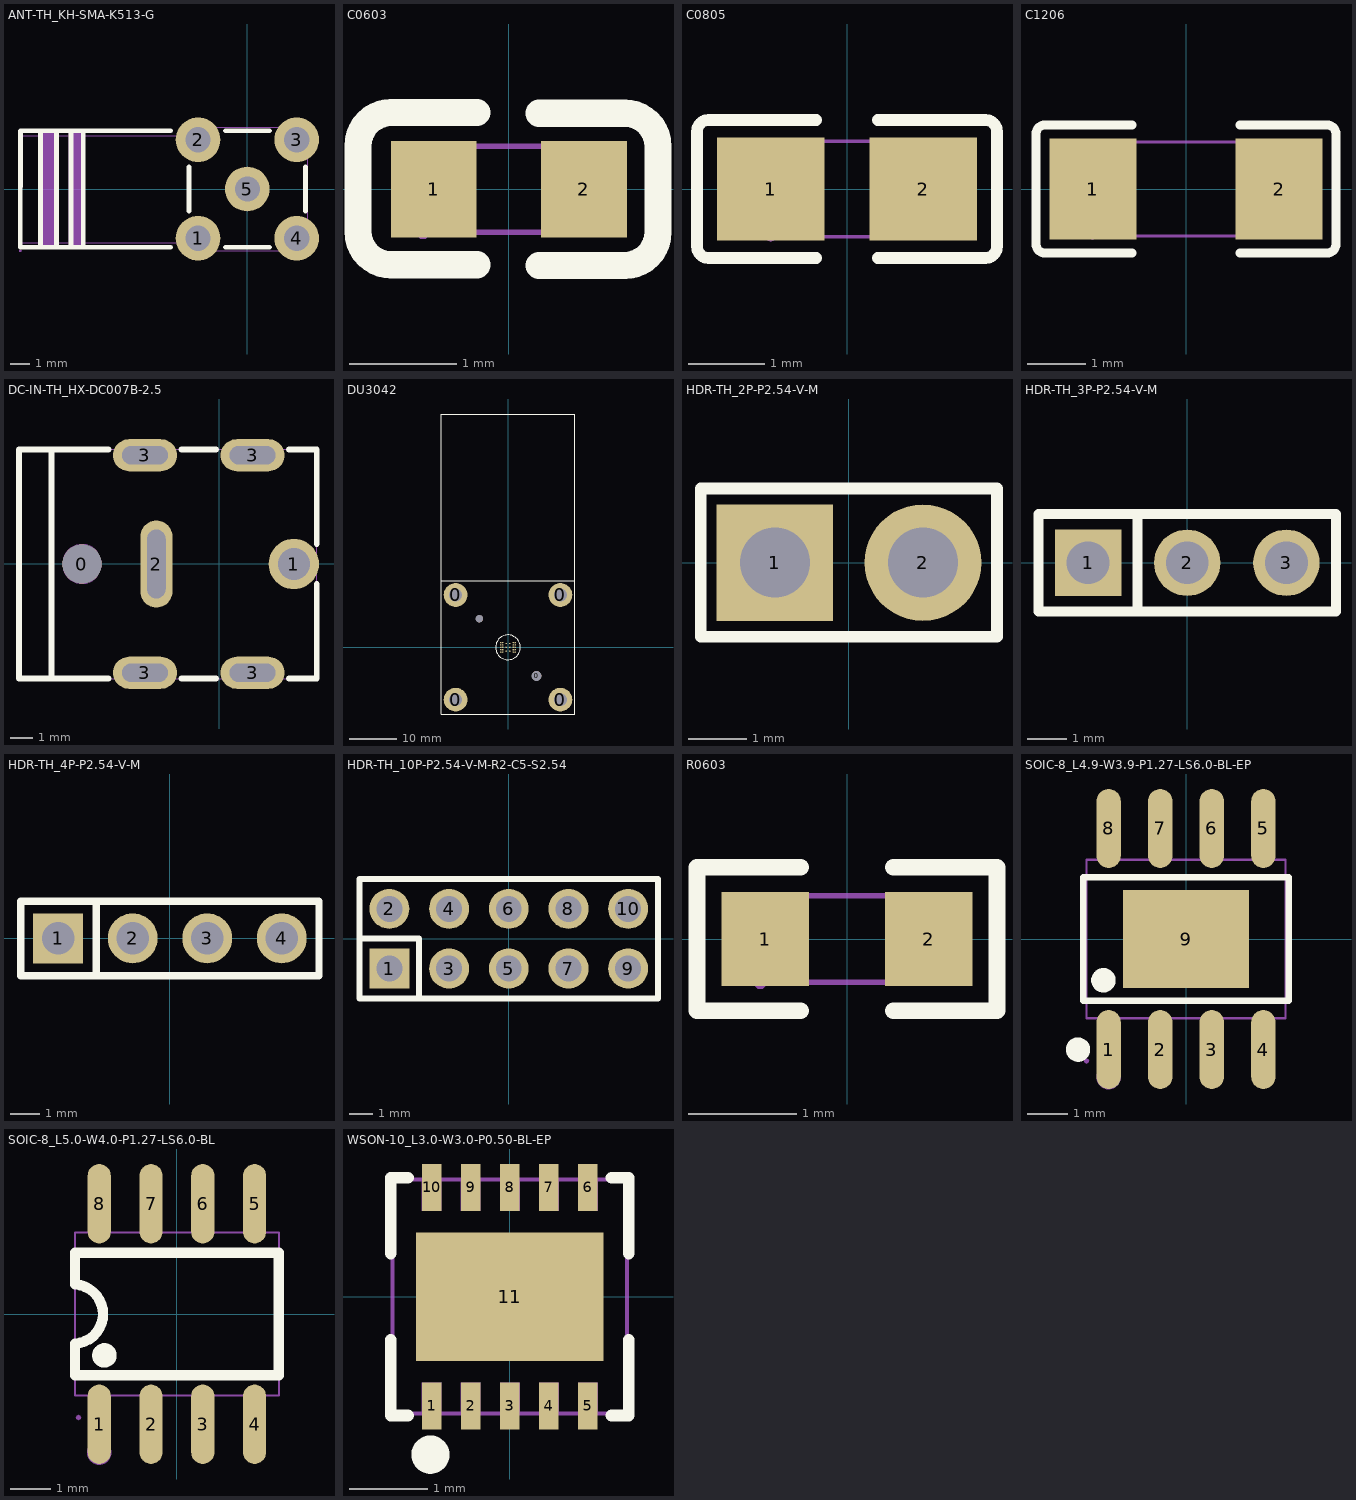
[diagram p0: the footprints below, top view; thin cyan lines are the x and y axes]
# Altium footprint library MISC75514.PcbLib: 14 footprints
Each footprint in its own frame and in the unit in brackets; x right, y up, seen from the top. Pads: shape width x height; smd on the part's side, far side on the other; paste and mask are expansions set on the pad; w line width, h text height; cw(c..) or ccw(c..) is an arc to the next point about the centre after c.

## ANT-TH_KH-SMA-K513-G [mm]
height 1.4
pads (5):
  round 2.3 hole 1.3 paste+0.051: 1(-2.54,-2.54) 2(-2.54,2.54) 3(2.54,2.54) 4(2.54,-2.54) 5(0,0)
Top Overlay:
  lines w0.254: -11.69,2.98 -11.7,-2.83 -11.7,-3 -11.5,-3 -3.948,-3 ; -11.69,3 -11.361,3 ; -11.5,3 -3.948,3 ; -10.668,-3 -10.668,3 ; -9.966,3 -9.573,3 ; -9.827,-3 -9.827,3 ; -9.09,-3 -9.09,3 ; -8.595,3 -8.176,3 ; -8.455,-3 -8.455,3 ; -3,-1.132 -3,1.132 ; -1.132,-3 1.132,-3 ; -1.132,3 1.132,3 ; 3,-1.132 3,1.132
Mechanical 2:
  region: -9.194,2.972 -8.394,2.972 -8.394,-3.018 -8.404,-3.028 -9.204,-3.028
  region: -10.64,3 -9.84,3 -9.84,-2.99 -9.85,-3 -10.65,-3
Mechanical 6:
  lines w0.051: -11.7,-2.76 -3.25,-2.76 -3.25,-3.17 3.1,-3.18 3.1,3.17 -3.25,3.17 -3.25,2.75 -11.7,2.75 -11.7,-2.76
Mechanical 8:
  region: -11.635,-3.18 -11.654,-3.226 -11.7,-3.245 -11.746,-3.226 -11.765,-3.18 -11.746,-3.134 -11.7,-3.115 -11.654,-3.134
Mechanical 9:
  region: -2.99,-2.09 -2.09,-2.09 -2.09,-2.99 -2.99,-2.99
  region: 2.09,2.99 2.99,2.99 2.99,2.09 2.09,2.09
  region: -2.99,2.99 -2.09,2.99 -2.09,2.09 -2.99,2.09
  region: 2.09,-2.09 2.99,-2.09 2.99,-2.99 2.09,-2.99
  region: 0.408,0 0.377,-0.156 0.288,-0.288 0.156,-0.377 0,-0.408 -0.156,-0.377 -0.288,-0.288 -0.377,-0.156 -0.408,0 -0.377,0.156 -0.288,0.288 -0.156,0.377 0,0.408 0.156,0.377 0.288,0.288 0.377,0.156

## C0603 [mm]
height 1.4
pads (2):
  rect 0.8x0.9 smd: 1(-0.7,0) 2(0.7,0)
Top Overlay:
  lines w0.254: -0.296,-0.704 -1.096,-0.704 cw(c-1.096,-0.394) -1.406,-0.394 -1.405,0.406 cw(c-1.096,0.406) -1.096,0.715 -0.296,0.715 ; 0.28,-0.71 1.08,-0.71 ccw(c1.08,-0.4) 1.39,-0.4 1.39,0.4 ccw(c1.08,0.4) 1.08,0.71 0.28,0.71
Mechanical 15:
  region: -0.8,-0.4 -0.8,0.4 -0.5,0.4 -0.5,-0.4
  region: 0.8,-0.4 0.8,0.4 0.5,0.4 0.5,-0.4
  region: -0.74,-0.4 -0.74,-0.375 -0.775,-0.341 -0.825,-0.341 -0.86,-0.375 -0.86,-0.4 -0.86,-0.425 -0.825,-0.459 -0.776,-0.459 -0.741,-0.425 -0.74,-0.4
  lines w0.051: -0.8,-0.4 -0.8,0.4 0.8,0.4 0.8,-0.4 -0.8,-0.4

## C0805 [mm]
height 1.4
pads (2):
  rect 1.41x1.35 smd paste-100 mask+0.051: 1(-1,0) 2(1,0)
Top Overlay:
  lines w0.152: -0.401,-0.904 -1.811,-0.904 cw(c-1.811,-0.751) -1.964,-0.751 -1.964,0.751 cw(c-1.811,0.751) -1.811,0.904 -0.401,0.904 ; 0.401,-0.904 1.811,-0.904 ccw(c1.811,-0.751) 1.964,-0.751 1.964,0.751 ccw(c1.811,0.751) 1.811,0.904 0.401,0.904
Top Paste:
  region: -1.705,-0.64 -1.705,0.64 -1.655,0.69 -0.505,0.69 -0.455,0.64 -0.45,0.23 -0.9,0.23 -0.9,-0.22 -0.46,-0.22 -0.455,-0.64 -0.505,-0.69 -1.655,-0.69
  region: 1.705,0.64 1.705,-0.64 1.655,-0.69 0.505,-0.69 0.455,-0.64 0.45,-0.23 0.9,-0.23 0.9,0.22 0.46,0.22 0.455,0.64 0.505,0.69 1.655,0.69
Mechanical 6:
  lines w0.051: -1,-0.625 -1,0.625 1,0.625 1,-0.625 -1,-0.625
Mechanical 8:
  region: -0.935,-0.625 -0.954,-0.671 -1,-0.69 -1.046,-0.671 -1.065,-0.625 -1.046,-0.579 -1,-0.56 -0.954,-0.579
Mechanical 9:
  region: -1,-0.625 -1,0.625 -0.5,0.625 -0.5,-0.625
  region: 1,0.625 1,-0.625 0.5,-0.625 0.5,0.625

## C1206 [mm]
height 1.4
pads (2):
  rect 1.485x1.728 smd paste-100 mask+0.051: 1(-1.593,0) 2(1.593,0)
Top Overlay:
  lines w0.152: -0.926,-1.093 -2.411,-1.093 cw(c-2.411,-0.94) -2.564,-0.94 -2.564,0.94 cw(c-2.411,0.94) -2.411,1.093 -0.926,1.093 ; 0.926,-1.093 2.411,-1.093 ccw(c2.411,-0.94) 2.564,-0.94 2.564,0.94 ccw(c2.411,0.94) 2.411,1.093 0.926,1.093
Top Paste:
  region: 0.85,-0.764 0.85,-0.394 0.95,-0.294 1.255,-0.294 1.355,-0.194 1.355,0.194 1.255,0.294 0.95,0.294 0.85,0.394 0.85,0.764 0.95,0.864 2.235,0.864 2.335,0.764 2.335,-0.764 2.235,-0.864 0.95,-0.864
  region: -0.85,-0.764 -0.85,-0.394 -0.95,-0.294 -1.255,-0.294 -1.355,-0.194 -1.355,0.194 -1.255,0.294 -0.95,0.294 -0.85,0.394 -0.85,0.764 -0.95,0.864 -2.235,0.864 -2.335,0.764 -2.335,-0.764 -2.235,-0.864 -0.95,-0.864
Mechanical 6:
  lines w0.051: -1.6,-0.8 -1.6,0.8 1.6,0.8 1.6,-0.8 -1.6,-0.8
Mechanical 8:
  region: -1.535,-0.8 -1.554,-0.846 -1.6,-0.865 -1.646,-0.846 -1.665,-0.8 -1.646,-0.754 -1.6,-0.735 -1.554,-0.754
Mechanical 9:
  region: -1.6,-0.8 -1.6,0.8 -1.1,0.8 -1.1,-0.8
  region: 1.6,-0.8 1.6,0.8 1.1,0.8 1.1,-0.8

## DC-IN-TH_HX-DC007B-2.5 [mm]
height 1.4
pads (7):
  round 1.7 hole 1.7 unplated: 0(-6,0)
  round 2.2 hole 1.4: 1(3.25,0)
  oval 1.4x3.8 hole 0.8 slot 3 at 90 deg: 2(-2.75,0)
  oval 2.8x1.4 hole 0.8 slot 2 at 0 deg: 3(-3.25,-4.75) 3(-3.25,4.75) 3(1.45,-4.75) 3(1.45,4.75)
Top Overlay:
  lines w0.254: -7.325,-5 -7.325,5 ; -4.847,-5 -8.75,-5 -8.75,5 -4.847,5 ; -1.653,-5 -0.147,-5 ; -1.653,5 -0.147,5 ; 3.047,-5 4.25,-5 4.25,-0.877 ; 3.047,5 4.25,5 4.25,0.877
Mechanical 1:
  circle w0.005: c-6,0 r0.85
Mechanical 15:
  region: 4.31,-5 4.309,-4.976 4.274,-4.943 4.226,-4.943 4.191,-4.976 4.19,-5 4.191,-5.024 4.226,-5.058 4.274,-5.058 4.309,-5.024 4.31,-5
  region: -4.05,4.6 -4.05,4.9 -2.45,4.9 -2.45,4.6
  region: 0.65,4.6 0.65,4.9 2.25,4.9 2.25,4.6
  region: -4.05,-4.9 -4.05,-4.6 -2.45,-4.6 -2.45,-4.9
  region: 0.65,-4.9 0.65,-4.6 2.25,-4.6 2.25,-4.9
  region: -2.65,-0.8 -2.85,-0.8 -2.85,0.8 -2.65,0.8
  region: 3.85,0 3.85,0.119 3.759,0.34 3.59,0.509 3.369,0.6 3.131,0.6 2.91,0.509 2.741,0.34 2.65,0.119 2.65,0 2.65,-0.119 2.741,-0.34 2.91,-0.509 3.131,-0.6 3.369,-0.6 3.59,-0.509 3.759,-0.34 3.85,-0.119 3.85,0
  lines w0.051: -8.75,-5 4.25,-5 4.25,5 -8.75,5 -8.75,-5

## DU3042 [mm]
height 1.4
pads (32):
  round 5 hole 2.7: 0(-11,-11) 0(-11,11) 0(11,-11) 0(11,11)
  round 1.5 hole 1.6 unplated: 0(-6,6)
  round 2 hole 2.1 unplated: 0(6,-6)
  round 0.3 smd: 1(-1.5,1) 2(-1.5,0.5) 3(-1.5,0) 4(-1.5,-0.5) 5(-1.5,-1) 6(1.5,-1) 7(1.5,-0.5) 8(1.5,0) 9(1.5,0.5) 10(1.5,1) 11(-0.4,-0.8) 11(-0.4,0) 11(-0.4,0.8) 11(0.4,-0.8) 11(0.4,0) 11(0.4,0.8) NC(-1.1,-1) NC(-1.1,-0.5) NC(-1.1,0) NC(-1.1,0.5) NC(-1.1,1) NC(1.1,-1) NC(1.1,-0.5) NC(1.1,0) NC(1.1,0.5) NC(1.1,1)
Top Overlay:
  circle w0.127: c0,0 r2.6
  lines w0.127: -14,14 -14,49 14,49 14,14 ; -14,14 -14,-14 14,-14 14,14 ; -14,14 14,14

## HDR-TH_2P-P2.54-V-M [mm]
height 1.4
pads (2):
  rect 2x2 hole 1.2 paste+0.051: 1(-1.27,0)
  round 2 hole 1.2 paste+0.051: 2(1.27,0)
Top Overlay:
  lines w0.203: -2.54,-1.27 2.54,-1.27 2.54,1.27 -0.635,1.27 -2.54,1.27 -2.54,-1.27
Mechanical 6:
  lines w0.051: -2.54,-1.25 -2.54,1.25 2.54,1.25 2.54,-1.25 -2.54,-1.25
Mechanical 8:
  region: -2.475,-1.25 -2.494,-1.296 -2.54,-1.315 -2.586,-1.296 -2.605,-1.25 -2.586,-1.204 -2.54,-1.185 -2.494,-1.204
Mechanical 9:
  region: 0.95,0.32 1.59,0.32 1.59,-0.32 0.95,-0.32
  region: -1.59,0.32 -0.95,0.32 -0.95,-0.32 -1.59,-0.32

## HDR-TH_3P-P2.54-V-M [mm]
height 1.4
pads (3):
  rect 1.7x1.7 hole 1.1 paste+0.051: 1(-2.54,0)
  round 1.7 hole 1.1 paste+0.051: 2(0,0) 3(2.54,0)
Top Overlay:
  lines w0.254: -1.27,-1.25 -1.27,1.25 ; 3.809,-1.25 3.809,1.25 -3.81,1.25 -3.81,-1.25 3.81,-1.25
Mechanical 6:
  lines w0.051: -3.81,-1.25 -3.81,1.25 3.81,1.25 3.81,-1.25 -3.81,-1.25
Mechanical 8:
  region: -3.745,-1.25 -3.764,-1.296 -3.81,-1.315 -3.856,-1.296 -3.875,-1.25 -3.856,-1.204 -3.81,-1.185 -3.764,-1.204
Mechanical 9:
  region: 2.22,0.32 2.86,0.32 2.86,-0.32 2.22,-0.32
  region: -0.32,0.32 0.32,0.32 0.32,-0.32 -0.32,-0.32
  region: -2.86,0.32 -2.22,0.32 -2.22,-0.32 -2.86,-0.32

## HDR-TH_4P-P2.54-V-M [mm]
height 1.4
pads (4):
  rect 1.7x1.7 hole 1.1 paste+0.051: 1(-3.81,0)
  round 1.7 hole 1.1 paste+0.051: 2(-1.27,0) 3(1.27,0) 4(3.81,0)
Top Overlay:
  lines w0.254: -2.516,-1.27 -2.516,1.27 ; -2.516,1.27 5.08,1.27 5.08,-1.27 -5.08,-1.27 -5.08,1.27 -2.516,1.27
Mechanical 6:
  lines w0.051: -5.08,-1.25 -5.08,1.25 5.08,1.25 5.08,-1.25 -5.08,-1.25
Mechanical 8:
  region: -5.015,-1.25 -5.034,-1.296 -5.08,-1.315 -5.126,-1.296 -5.145,-1.25 -5.126,-1.204 -5.08,-1.185 -5.034,-1.204
Mechanical 9:
  region: -4.13,0.32 -3.49,0.32 -3.49,-0.32 -4.13,-0.32
  region: -1.59,0.32 -0.95,0.32 -0.95,-0.32 -1.59,-0.32
  region: 0.95,0.32 1.59,0.32 1.59,-0.32 0.95,-0.32
  region: 3.49,0.32 4.13,0.32 4.13,-0.32 3.49,-0.32

## HDR-TH_10P-P2.54-V-M-R2-C5-S2.54 [mm]
height 1.4
pads (10):
  rect 1.7x1.7 hole 1.1 paste+0.051: 1(-5.08,-1.27)
  round 1.7 hole 1.1 paste+0.051: 2(-5.08,1.27) 3(-2.54,-1.27) 4(-2.54,1.27) 5(0,-1.27) 6(0,1.27) 7(2.54,-1.27) 8(2.54,1.27) 9(5.08,-1.27) 10(5.08,1.27)
Top Overlay:
  lines w0.254: -6.35,0 -3.81,0.007 -3.81,-2.54 ; -6.35,-2.54 -6.35,2.54 6.35,2.54 6.35,-2.54 -6.35,-2.54
Mechanical 6:
  lines w0.051: -6.35,-2.5 6.35,-2.5 6.35,2.5 -6.35,2.5 -6.35,-2.5
Mechanical 8:
  region: -6.285,-2.5 -6.304,-2.546 -6.35,-2.565 -6.396,-2.546 -6.415,-2.5 -6.396,-2.454 -6.35,-2.435 -6.304,-2.454
Mechanical 9:
  region: 4.76,-0.95 5.4,-0.95 5.4,-1.59 4.76,-1.59
  region: 4.76,1.59 5.4,1.59 5.4,0.95 4.76,0.95
  region: 2.22,-0.95 2.86,-0.95 2.86,-1.59 2.22,-1.59
  region: 2.22,1.59 2.86,1.59 2.86,0.95 2.22,0.95
  region: -0.32,-0.95 0.32,-0.95 0.32,-1.59 -0.32,-1.59
  region: -0.32,1.59 0.32,1.59 0.32,0.95 -0.32,0.95
  region: -2.86,-0.95 -2.22,-0.95 -2.22,-1.59 -2.86,-1.59
  region: -2.86,1.59 -2.22,1.59 -2.22,0.95 -2.86,0.95
  region: -5.4,-0.95 -4.76,-0.95 -4.76,-1.59 -5.4,-1.59
  region: -5.4,1.59 -4.76,1.59 -4.76,0.95 -5.4,0.95

## R0603 [mm]
height 1.4
pads (2):
  rect 0.806x0.864 smd paste-100 mask+0.051: 1(-0.753,0) 2(0.753,0)
Top Overlay:
  lines w0.152: -0.426,-0.661 -1.385,-0.661 -1.385,0.661 -0.426,0.661 ; 0.426,-0.661 1.385,-0.661 1.385,0.661 0.426,0.661
Top Paste:
  region: 1.195,0.45 0.395,0.45 0.345,0.4 0.345,0.172 0.715,0.172 0.715,-0.158 0.345,-0.158 0.345,-0.4 0.395,-0.45 1.195,-0.45 1.245,-0.4 1.245,0.4
  region: -0.355,0.4 -0.355,0.172 -0.735,0.172 -0.735,-0.158 -0.355,-0.158 -0.355,-0.4 -0.405,-0.45 -1.195,-0.45 -1.245,-0.4 -1.245,0.4 -1.195,0.45 -0.405,0.45
Mechanical 15:
  region: -0.8,-0.4 -0.8,0.4 -0.5,0.4 -0.5,-0.4
  region: 0.8,-0.4 0.8,0.4 0.5,0.4 0.5,-0.4
  region: -0.74,-0.4 -0.741,-0.376 -0.776,-0.342 -0.824,-0.342 -0.859,-0.376 -0.86,-0.4 -0.859,-0.424 -0.825,-0.458 -0.776,-0.458 -0.741,-0.424 -0.74,-0.4
  lines w0.051: -0.8,-0.4 -0.8,0.4 0.8,0.4 0.8,-0.4 -0.8,-0.4

## SOIC-8_L4.9-W3.9-P1.27-LS6.0-BL-EP [mm]
height 1.4
pads (9):
  oval 0.602x1.941 smd paste+0.051: 1(-1.905,-2.721) 2(-0.635,-2.721) 3(0.635,-2.721) 4(1.905,-2.721) 5(1.905,2.721) 6(0.635,2.721) 7(-0.635,2.721) 8(-1.905,2.721)
  rect 3.098x2.41 smd paste+0.051: 9(0,0)
Top Overlay:
  circle w0.3: c-2.032,-1.016 r0.15
  circle w0.3: c-2.658,-2.721 r0.15
  lines w0.152: -2.526,-1.521 -2.526,1.521 2.526,1.521 2.526,-1.521 -2.526,-1.521
Mechanical 2:
  circle w0.3: c-1.905,-3.4 r0.15
Mechanical 6:
  lines w0.051: -2.45,-1.95 -2.45,1.95 2.45,1.95 2.45,-1.95 -2.45,-1.95
Mechanical 7:
  region: -2.12,-2.36 -2.12,-1.94 -1.69,-1.94 -1.69,-2.36
  region: -0.85,-2.36 -0.85,-1.94 -0.42,-1.94 -0.42,-2.36
  region: 0.42,-2.36 0.42,-1.94 0.85,-1.94 0.85,-2.36
  region: 1.69,-2.36 1.69,-1.94 2.12,-1.94 2.12,-2.36
  region: -2.12,2.36 -2.12,1.94 -1.69,1.94 -1.69,2.36
  region: -0.85,2.36 -0.85,1.94 -0.42,1.94 -0.42,2.36
  region: 0.42,2.36 0.42,1.94 0.85,1.94 0.85,2.36
  region: 1.69,2.36 1.69,1.94 2.12,1.94 2.12,2.36
Mechanical 8:
  region: -2.385,-3 -2.404,-3.046 -2.45,-3.065 -2.496,-3.046 -2.515,-3 -2.496,-2.954 -2.45,-2.935 -2.404,-2.954
Mechanical 9:
  region: -2.12,-3 -2.12,-2.35 -1.69,-2.35 -1.69,-3
  region: -0.85,-3 -0.85,-2.35 -0.42,-2.35 -0.42,-3
  region: 0.42,-3 0.42,-2.35 0.85,-2.35 0.85,-3
  region: 1.69,-3 1.69,-2.35 2.12,-2.35 2.12,-3
  region: -2.12,3 -2.12,2.35 -1.69,2.35 -1.69,3
  region: -0.85,3 -0.85,2.35 -0.42,2.35 -0.42,3
  region: 0.42,3 0.42,2.35 0.85,2.35 0.85,3
  region: 1.69,3 1.69,2.35 2.12,2.35 2.12,3
  region: -1.549,1.205 1.549,1.205 1.549,-1.205 -1.549,-1.205

## SOIC-8_L5.0-W4.0-P1.27-LS6.0-BL [mil]
height 55.12
pads (8):
  oval 22.38x76.78 smd paste+2: 1(-75,-106.5) 2(-25,-106.5) 3(25,-106.5) 4(75,-106.5) 5(75,106.5) 6(25,106.5) 7(-25,106.5) 8(-75,106.5)
Top Overlay:
  circle w11.81: c-70,-40 r5.91
  lines w10: -98.43,-28.61 ccw(c-99.99,0) -98.23,28.59 ; -98.42,-28.61 -98.42,-59.05 98.42,-59.05 98.42,59.05 -98.42,59.05 -98.42,28.59
Mechanical 2:
  circle w11.81: c-75,-133.86 r5.91
Mechanical 6:
  lines w2: -98.42,-78.74 -98.42,78.74 98.42,78.74 98.42,-78.74 -98.42,-78.74
Mechanical 7:
  region: 66.93,76.38 66.93,85.63 83.07,85.63 83.07,76.38
  region: 16.93,76.38 16.93,85.63 33.07,85.63 33.07,76.38
  region: -33.07,76.38 -33.07,85.63 -16.93,85.63 -16.93,76.38
  region: -83.07,76.38 -83.07,85.63 -66.93,85.63 -66.93,76.38
  region: 66.93,-85.63 66.93,-76.38 83.07,-76.38 83.07,-85.63
  region: 16.93,-85.63 16.93,-76.38 33.07,-76.38 33.07,-85.63
  region: -33.07,-85.63 -33.07,-76.38 -16.93,-76.38 -16.93,-85.63
  region: -83.07,-85.63 -83.07,-76.38 -66.93,-76.38 -66.93,-85.63
Mechanical 8:
  region: -92.44,-100 -93.19,-101.81 -95,-102.56 -96.81,-101.81 -97.56,-100 -96.81,-98.19 -95,-97.44 -93.19,-98.19
Mechanical 9:
  region: 66.93,85.24 66.93,118.11 83.07,118.11 83.07,85.24
  region: 16.93,85.24 16.93,118.11 33.07,118.11 33.07,85.24
  region: -33.07,85.24 -33.07,118.11 -16.93,118.11 -16.93,85.24
  region: -83.07,85.24 -83.07,118.11 -66.93,118.11 -66.93,85.24
  region: 66.93,-118.11 66.93,-85.24 83.07,-85.24 83.07,-118.11
  region: 16.93,-118.11 16.93,-85.24 33.07,-85.24 33.07,-118.11
  region: -33.07,-118.11 -33.07,-85.24 -16.93,-85.24 -16.93,-118.11
  region: -83.07,-118.11 -83.07,-85.24 -66.93,-85.24 -66.93,-118.11

## WSON-10_L3.0-W3.0-P0.50-BL-EP [mm]
height 1.4
pads (11):
  rect 0.25x0.6 smd paste+0.051: 1(-1.001,-1.4) 2(-0.5,-1.4) 3(0,-1.4) 4(0.5,-1.4) 5(1.001,-1.4) 6(1.001,1.4) 7(0.5,1.4) 8(0,1.4) 9(-0.5,1.4) 10(-1.001,1.4)
  rect 2.4x1.65 smd paste+0.051: 11(0,0)
Top Overlay:
  lines w0.15: -1.524,-0.554 -1.524,-1.524 -1.305,-1.524 ; -1.524,0.554 -1.524,1.524 -1.305,1.524 ; 1.305,-1.524 1.524,-1.524 1.524,-0.554 ; 1.305,1.524 1.524,1.524 1.524,0.554
  lines w0.25: -1.019,-1.905 ccw(c-1.017,-2.025) -1.016,-1.905
Mechanical 6:
  lines w0.051: -1.5,-1.5 -1.5,1.5 1.5,1.5 1.5,-1.5 -1.5,-1.5
Mechanical 8:
  region: -1.439,-1.502 -1.458,-1.548 -1.504,-1.567 -1.55,-1.548 -1.569,-1.502 -1.55,-1.456 -1.504,-1.437 -1.458,-1.456
Mechanical 9:
  region: -1.126,1.501 -0.876,1.501 -0.876,1.101 -1.126,1.101
  region: -0.625,1.501 -0.375,1.501 -0.375,1.101 -0.625,1.101
  region: -0.125,1.501 0.125,1.501 0.125,1.101 -0.125,1.101
  region: 0.375,1.501 0.625,1.501 0.625,1.101 0.375,1.101
  region: 0.876,1.501 1.126,1.501 1.126,1.101 0.876,1.101
  region: -0.876,-1.501 -1.126,-1.501 -1.126,-1.101 -0.876,-1.101
  region: -0.375,-1.501 -0.625,-1.501 -0.625,-1.101 -0.375,-1.101
  region: 0.125,-1.501 -0.125,-1.501 -0.125,-1.101 0.125,-1.101
  region: 0.625,-1.501 0.375,-1.501 0.375,-1.101 0.625,-1.101
  region: 1.126,-1.501 0.876,-1.501 0.876,-1.101 1.126,-1.101